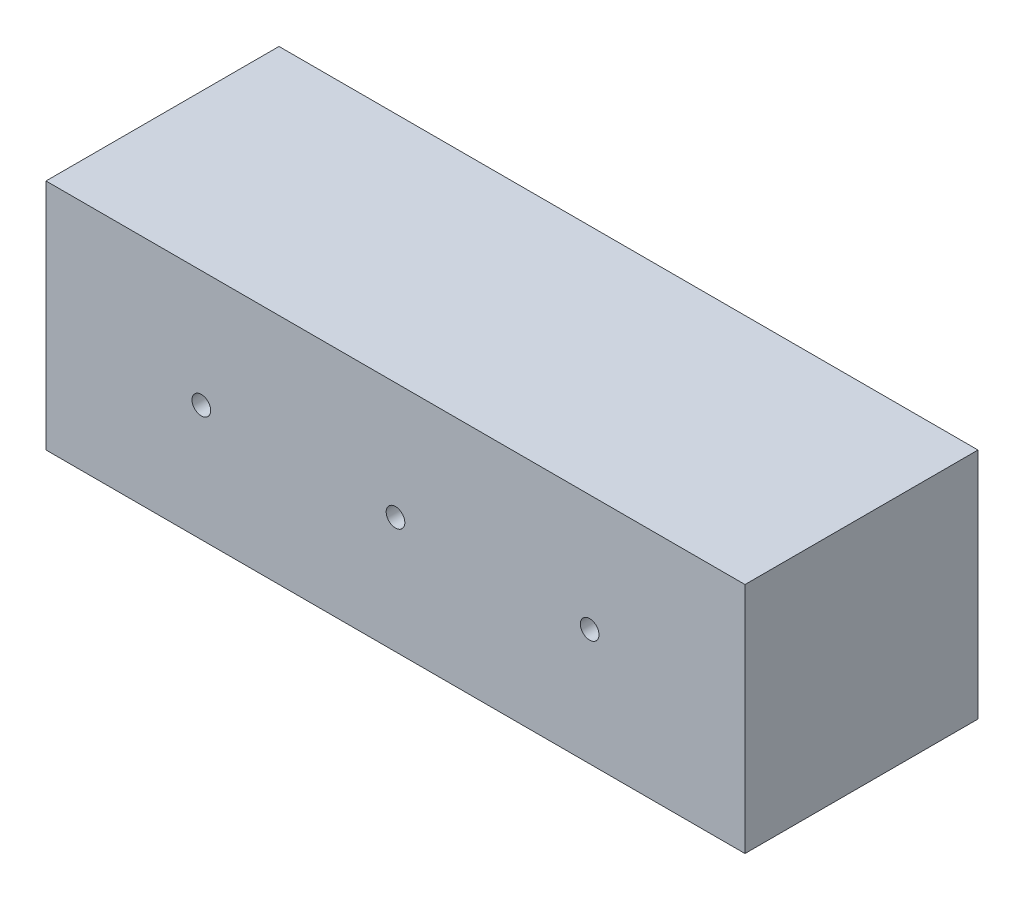
from build123d import *

# Parameters (mm, degrees)
SKETCH_1_W         = 180
SKETCH_1_H         = 60
EXTRUDE_1_DEPTH    = 60
HOLE_WIZARD_M4_1_D = 4.8


with BuildPart() as part:
    # 草图1 → 凸台-拉伸1 (new body)
    with BuildSketch(Plane(origin=(0, 0, 0), x_dir=(1, 0, 0), z_dir=(0, 1, 0))):
        Rectangle(SKETCH_1_W, SKETCH_1_H)
    extrude(amount=EXTRUDE_1_DEPTH)

    # M4 间隙孔1 (through all)
    with Locations(Plane(origin=(0, 0, -30), x_dir=(-1, 0, 0), z_dir=(0, 0, -1))):
        with Locations((0, 30), (50, 30), (-50, 30)):
            Hole(HOLE_WIZARD_M4_1_D / 2)


solid = part.part
